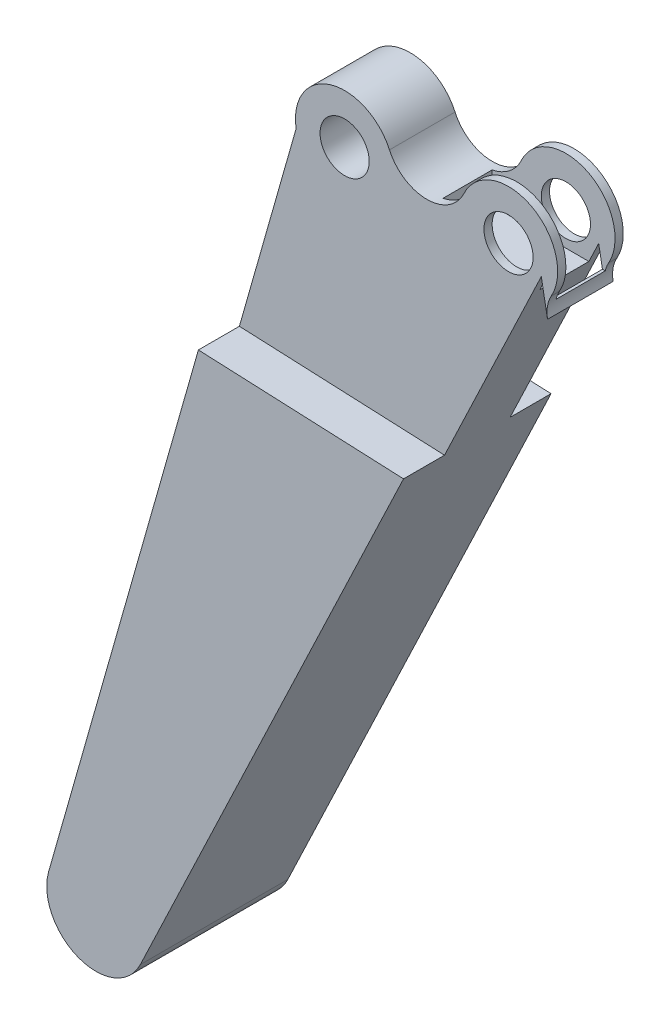
from build123d import *

# Parameters (mm, degrees)
SKETCH1_R               = 3
BOSS_EXTRUDE1_DEPTH     = 8
CUT_EXTRUDE1_DEPTH      = 10
CUT_EXTRUDE1_DEPTH_BACK = 10
SKETCH2_W               = 30
SKETCH2_H               = 6
BOSS_EXTRUDE2_DEPTH     = 5
SCALE1_SCALE            = 0.5


with BuildPart() as part:
    # Sketch1 → Boss-Extrude1 (new body)
    with BuildSketch(Plane.XY):
        with BuildLine():
            Line((-59.466854234, -95.453658304), (-34.265346163, -6.824512068))
            ThreePointArc((-34.265346163, -6.824512068), (-30.086435736, -0.093123284), (-22.875098798, -3.375120677))
            ThreePointArc((-22.875098798, -3.375120677), (-18.350652777, -6.324611935), (-13.784422872, -3.44023073))
            ThreePointArc((-13.784422872, -3.44023073), (-5.593314668, -0.648514381), (-3.132391837, -8.945007172))
            ThreePointArc((-3.132391837, -8.945007172), (-3.598758132, -10.251856882), (-3.590598772, -11.639404038))
            Line((-3.590598772, -11.639404038), (-4.345412305, -7.496284288))
            Line((-4.345412305, -7.496284288), (-48.279353466, -99.676151096))
            ThreePointArc((-48.279353466, -99.676151096), (-55.814324496, -102.708171614), (-59.466854234, -95.453658304))
        make_face()
        with Locations((-28.347406658, -5.835577277)):
            Circle(SKETCH1_R, mode=Mode.SUBTRACT)
        with Locations((-8.347919622, -5.978819396)):
            Circle(SKETCH1_R, mode=Mode.SUBTRACT)
    extrude(amount=BOSS_EXTRUDE1_DEPTH)

    # Sketch2 → Cut-Extrude1 (cut, two sides: drawn at the far end of the back side and taken through both)
    with BuildSketch(Plane(origin=(0, 0, 0), x_dir=(1, 0, 0), z_dir=(0, 1, 0)).offset(-CUT_EXTRUDE1_DEPTH_BACK)):
        with Locations((-2.347919622, -4)):
            Rectangle(SKETCH2_W, SKETCH2_H)
    extrude(amount=CUT_EXTRUDE1_DEPTH + CUT_EXTRUDE1_DEPTH_BACK, mode=Mode.SUBTRACT)

    # Sketch3 → Boss-Extrude2 (add)
    with BuildSketch(Plane.XY.offset(8)):
        with BuildLine():
            Line((-16.158374435, -32.281615332), (-41.189011455, -31.173790769))
            Line((-41.189011455, -31.173790769), (-59.466854234, -95.453658304))
            ThreePointArc((-59.466854234, -95.453658304), (-55.814324496, -102.708171614), (-48.279353466, -99.676151096))
            Line((-48.279353466, -99.676151096), (-16.158374435, -32.281615332))
        make_face()
    boss_extrude2 = extrude(amount=BOSS_EXTRUDE2_DEPTH)

    # Mirror1: Boss-Extrude2 across plane
    add(boss_extrude2.mirror(Plane.XY.offset(4)))


with BuildPart() as part_1:
    # Scale1: scaled about (0, 0, 0)
    add(part.part.scale(SCALE1_SCALE))


solid = part_1.part
